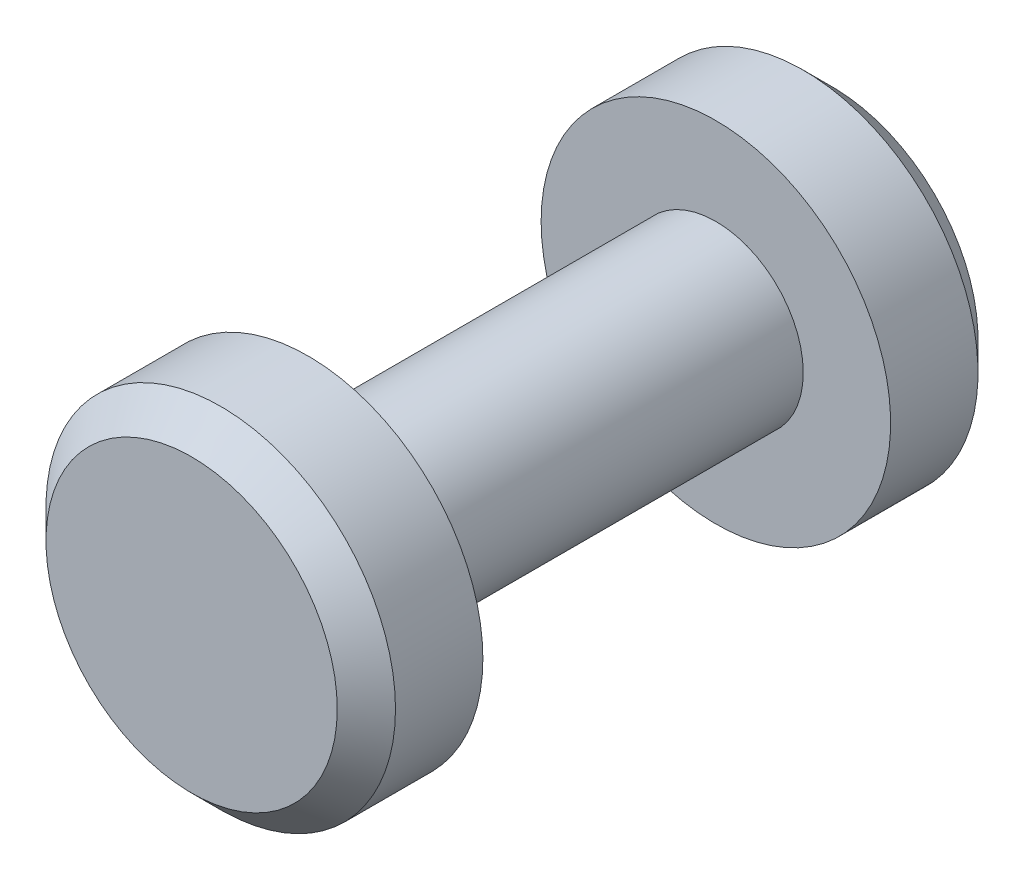
SolidWorks part; units mm, degrees
ref_plane "前视基准面" through (0, 0, 0) normal (0, 0, 1) x (1, 0, 0)
ref_plane "上视基准面" through (0, 0, 0) normal (0, 1, 0) x (1, 0, 0)
ref_plane "右视基准面" through (0, 0, 0) normal (1, 0, 0) x (0, 0, -1)
sketch "草图1" plane through (0, 0, 0) normal (0, 0, 1) x (1, 0, 0)
  circle A0 centre (0, 0) radius 3
extrude "凸台-拉伸1" add sketch "草图1" along normal blind 14
sketch "草图2" plane through (0, 0, 14) normal (0, 0, 1) x (1, 0, 0)
  circle A0 centre (0, 0) radius 6
extrude "凸台-拉伸2" add sketch "草图2" along normal blind 4
chamfer "倒角1" distance 1 angle 45 1 edges at (6, 0, 18)
sketch "草图3" plane through (0, 0, 0) normal (0, 0, -1) x (-1, 0, 0)
  circle A0 centre (0, 0) radius 6
extrude "凸台-拉伸3" add sketch "草图3" along normal blind 4
chamfer "倒角2" distance 1 angle 45 1 edges at (-6, 0, -4)
